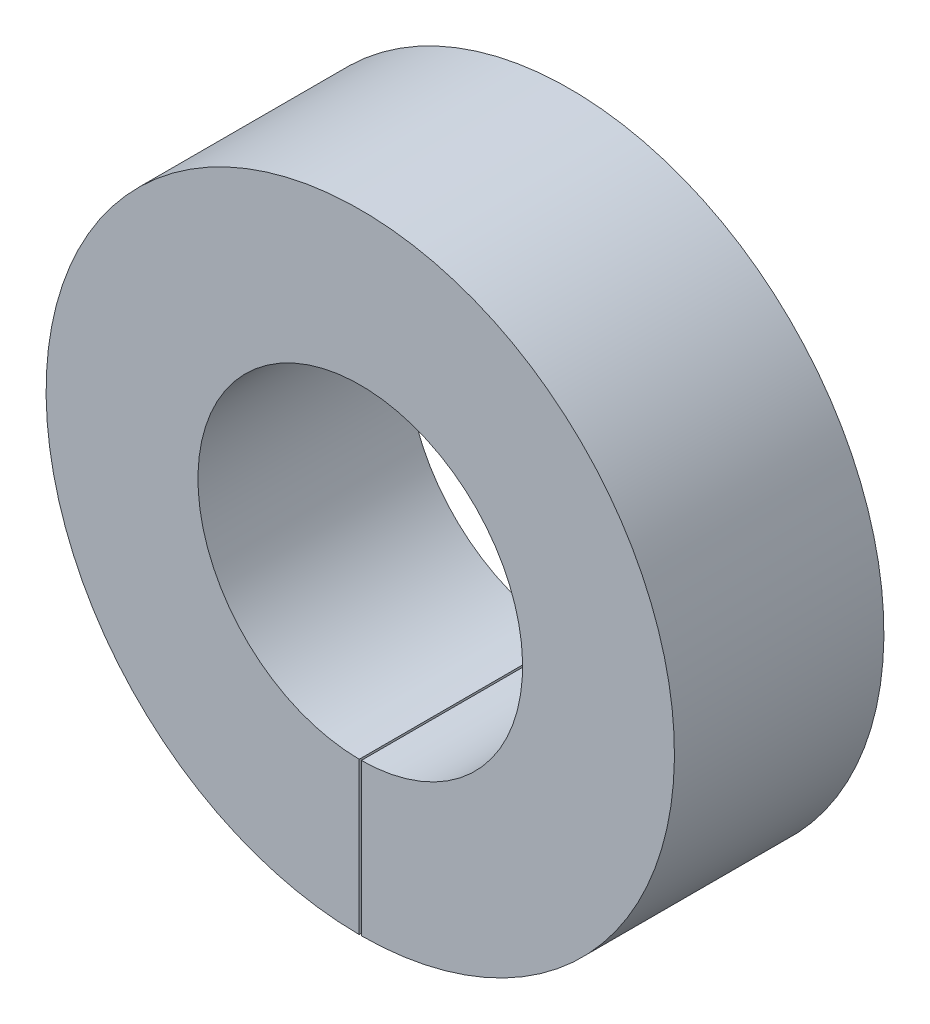
SolidWorks part; units mm, degrees
ref_plane "Front Plane" through (0, 0, 0) normal (0, 0, 1) x (1, 0, 0)
ref_plane "Top Plane" through (0, 0, 0) normal (0, 1, 0) x (1, 0, 0)
ref_plane "Right Plane" through (0, 0, 0) normal (1, 0, 0) x (0, 0, -1)
sketch "Sketch1" plane through (0, 0, 0) normal (0, 0, 1) x (1, 0, 0)
  circle A0 centre (0, 0) radius 7.75
  circle A1 centre (0, 0) radius 15
  dimension "D1" = 30
  dimension "D2" = 15.5
extrude "Boss-Extrude1" add sketch "Sketch1" along normal blind 10
sketch "Sketch2" plane through (0, 0, 10) normal (0, 0, 1) x (1, 0, 0)
  line L1 (-0.05, 3.4843) -> (0.05, 3.4843)
  line L2 (-0.05, 3.4843) -> (-0.05, -18.9843)
  line L3 (-0.05, -18.9843) -> (0.05, -18.9843)
  line L4 (0.05, 3.4843) -> (0.05, -18.9843)
  line L5 (-0.05, 3.4843) -> (0.05, -18.9843) construction
  line L6 (-0.05, -18.9843) -> (0.05, 3.4843) construction
  circle A0 centre (0, 0) radius 7.75 construction
  point P0 (0, -7.75)
  dimension "D1" = 0.1
extrude "Cut-Extrude1" cut sketch "Sketch2" against normal through all
